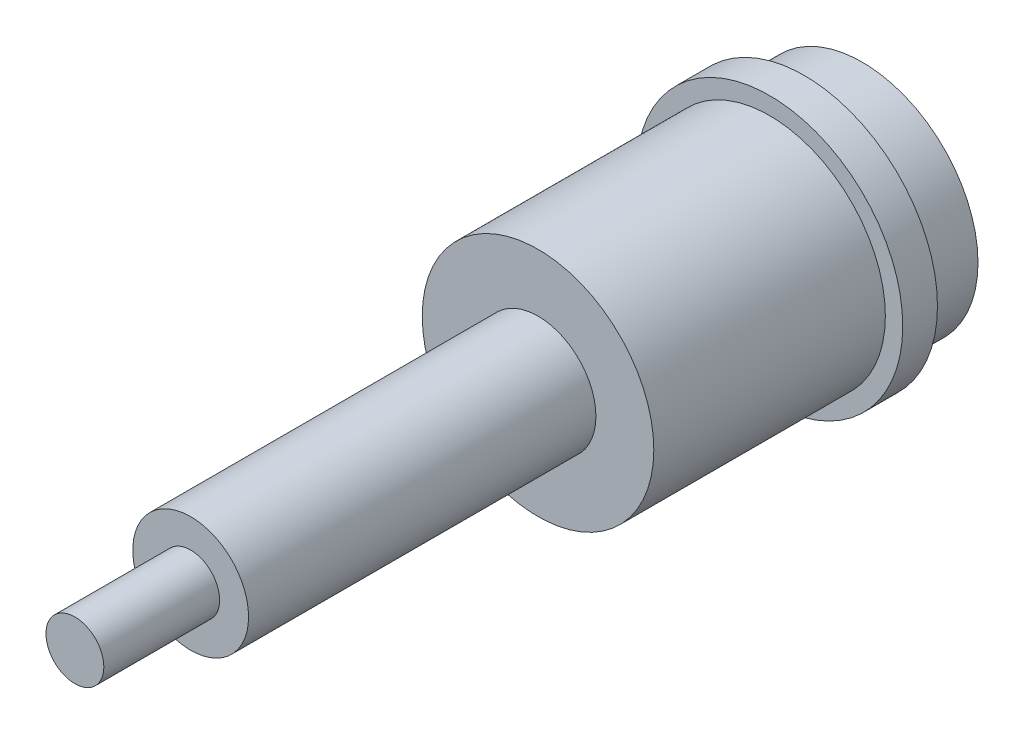
from build123d import *

# Parameters (mm, degrees)
SKETCH1_R           = 10
BOSS_EXTRUDE1_DEPTH = 5
SKETCH2_R           = 11.5
BOSS_EXTRUDE2_DEPTH = 3
SKETCH3_R           = 10
BOSS_EXTRUDE3_DEPTH = 20
SKETCH4_R           = 5
BOSS_EXTRUDE4_DEPTH = 30
SKETCH5_R           = 2.5
BOSS_EXTRUDE5_DEPTH = 10


with BuildPart() as part:
    # Sketch1 → Boss-Extrude1 (new body)
    with BuildSketch(Plane.XY):
        Circle(SKETCH1_R)
    extrude(amount=BOSS_EXTRUDE1_DEPTH)

    # Sketch2 → Boss-Extrude2 (add)
    with BuildSketch(Plane.XY.offset(5)):
        Circle(SKETCH2_R)
    extrude(amount=BOSS_EXTRUDE2_DEPTH)

    # Sketch3 → Boss-Extrude3 (add)
    with BuildSketch(Plane.XY.offset(8)):
        Circle(SKETCH3_R)
    extrude(amount=BOSS_EXTRUDE3_DEPTH)

    # Sketch4 → Boss-Extrude4 (add)
    with BuildSketch(Plane.XY.offset(28)):
        Circle(SKETCH4_R)
    extrude(amount=BOSS_EXTRUDE4_DEPTH)

    # Sketch5 → Boss-Extrude5 (add)
    with BuildSketch(Plane.XY.offset(58)):
        Circle(SKETCH5_R)
    extrude(amount=BOSS_EXTRUDE5_DEPTH)


solid = part.part
